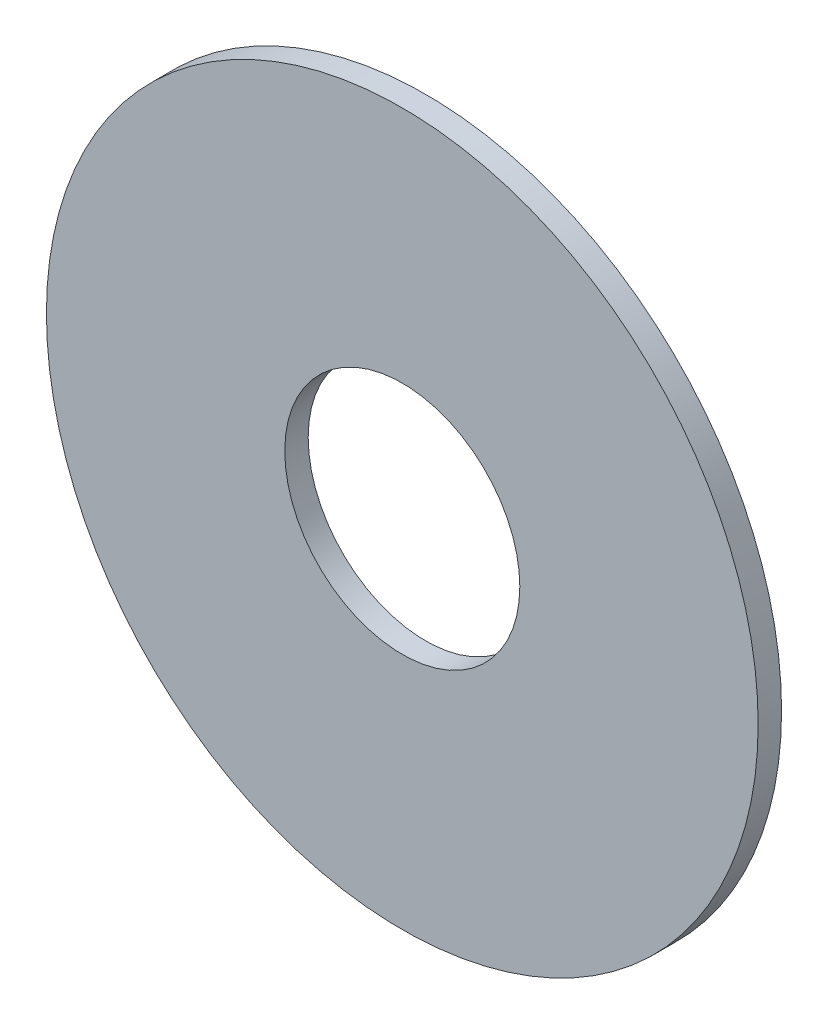
SolidWorks part; units mm, degrees
material "Q235B"
ref_plane "Front Plane" through (0, 0, 0) normal (0, 0, 1) x (1, 0, 0)
ref_plane "Top Plane" through (0, 0, 0) normal (0, 1, 0) x (1, 0, 0)
ref_plane "Right Plane" through (0, 0, 0) normal (1, 0, 0) x (0, 0, -1)
sketch "Sketch1" plane through (0, 0, 0) normal (0, 0, 1) x (1, 0, 0)
  circle A0 centre (0, 0) radius 62.75
  circle A1 centre (0, 0) radius 190
  dimension "D1" = 125.5
  dimension "D2" = 380
extrude "Boss-Extrude1" add sketch "Sketch1" along normal blind 12.5
